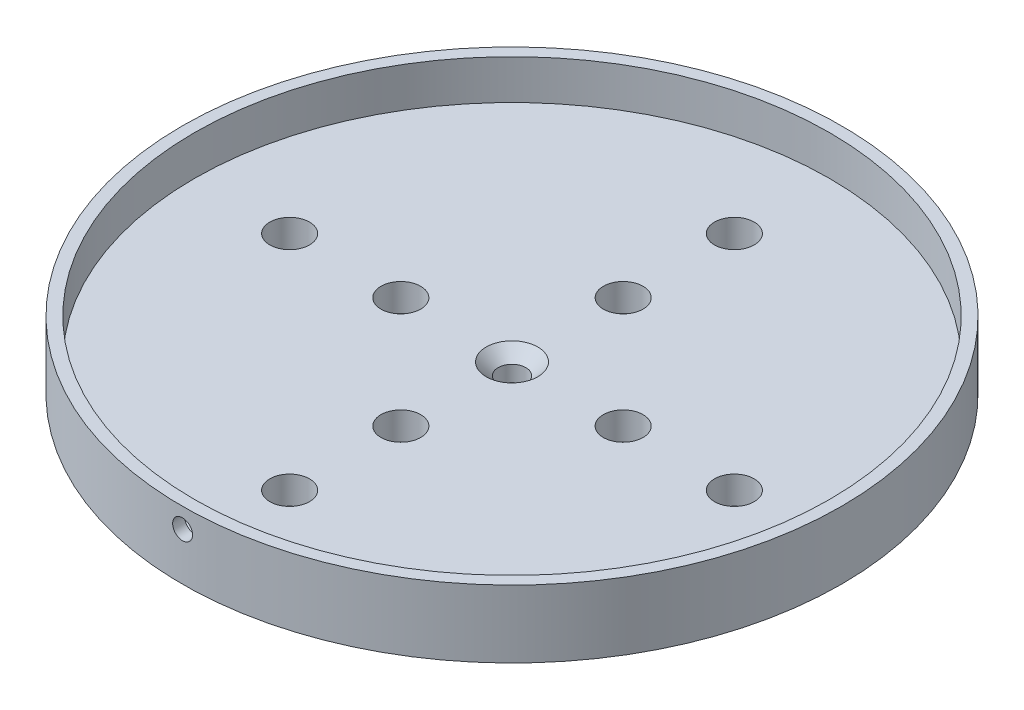
SolidWorks part; units mm, degrees
material "6061 合金"
ref_plane "Front Plane" through (0, 0, 0) normal (0, 0, 1) x (1, 0, 0)
ref_plane "Top Plane" through (0, 0, 0) normal (0, 1, 0) x (1, 0, 0)
ref_plane "Right Plane" through (0, 0, 0) normal (1, 0, 0) x (0, 0, -1)
sketch "Sketch1" plane through (0, 0, 0) normal (0, 0, 1) x (1, 0, 0)
  line L0 (0, 9.3101) -> (0, -2.1203) construction
  line L1 (1.75, 0) -> (1.75, 2)
  line L2 (3.25, 3.5) -> (40, 3.5)
  line L3 (40, 3.5) -> (40, 8.5)
  line L4 (40, 8.5) -> (41.5, 8.5)
  line L5 (41.5, 8.5) -> (41.5, 0)
  line L6 (41.5, 0) -> (1.75, 0)
  line L7 (1.75, 2) -> (3.25, 3.5)
  dimension "D1" = 1.75
  dimension "D2" = 41.5
  dimension "D3" = 40
  dimension "D4" = 5
  dimension "D5" = 8.5
  dimension "D6" = 135
  dimension "D7" = 3.25
revolve "Revolve1" add sketch "Sketch1" angle 360 about L0
sketch "Sketch2" plane through (0, 3.5, 0) normal (0, 1, 0) x (1, 0, 0)
  line L0 (0, 47.3195) -> (0, -44.9935) construction
  line L1 (-18.0109, 0) -> (13.536, 0) construction
  circle A0 centre (0, 14) radius 2.5
  circle A1 centre (14, 0) radius 2.5
  circle A2 centre (0, 28) radius 2.5
  circle A3 centre (28, 0) radius 2.5
  circle A4 centre (0, -14) radius 2.5
  circle A5 centre (0, -28) radius 2.5
  circle A6 centre (-14, 0) radius 2.5
  circle A7 centre (-28, 0) radius 2.5
  circle A8 centre (0, 0) radius 14 construction
  circle A9 centre (0, 0) radius 28 construction
  point P24 (0, 0)
  point P32 (0, 0.6519)
  dimension "D1" = 5
  dimension "D2" = 4
  dimension "D3" = 14
  dimension "D4" = 14
  dimension "D5" = 28
  dimension "D6" = 5
  dimension "D7" = 56
extrude "Cut-Extrude1" cut sketch "Sketch2" against normal up to next
chamfer "Chamfer1" [suppressed] distance 0.3 angle 45
ref_plane "Plane1" through (0, 0, 41.5) normal (0, 0, 1) x (1, 0, 0)
sketch "Sketch3" plane through (0, 0, 41.5) normal (0, 0, 1) x (1, 0, 0)
  line L0 (0, 0) -> (0, 8.5) construction
  line L1 (40, 8.5) -> (-40, 8.5) construction
  line L2 (41.5, 8.5) -> (-41.5, 8.5) construction
  circle A0 centre (0, 6) radius 1.5
  dimension "D1" = 3
  dimension "D2" = 2.5
hole_wizard "M3 Tapped Hole1" positions "3DSketch1" profile "Sketch4" tap size "M3" standard "GB"
sketch3d "3DSketch1"
  point P3 (0, 6, 41.5)
sketch "Sketch4" plane through (0, 6, 41.5) normal (1, 0, 0) x (0, -1, 0)
  line L0 (0, 0) -> (0, 1.5)
  line L1 (0, 1.5) -> (1.25, 1.5)
  line L2 (1.25, 1.5) -> (1.25, 0)
  line L5 (1.25, 0) -> (0, 0)
  line L11 (0, -6.35) -> (0, 107.95) construction
  dimension "通孔螺纹孔钻头直径" = 2.5
  dimension "通孔螺纹孔钻头深度" = 1.5
cosmetic thread "Cosmetic Thread3" parameters "D2"=3
